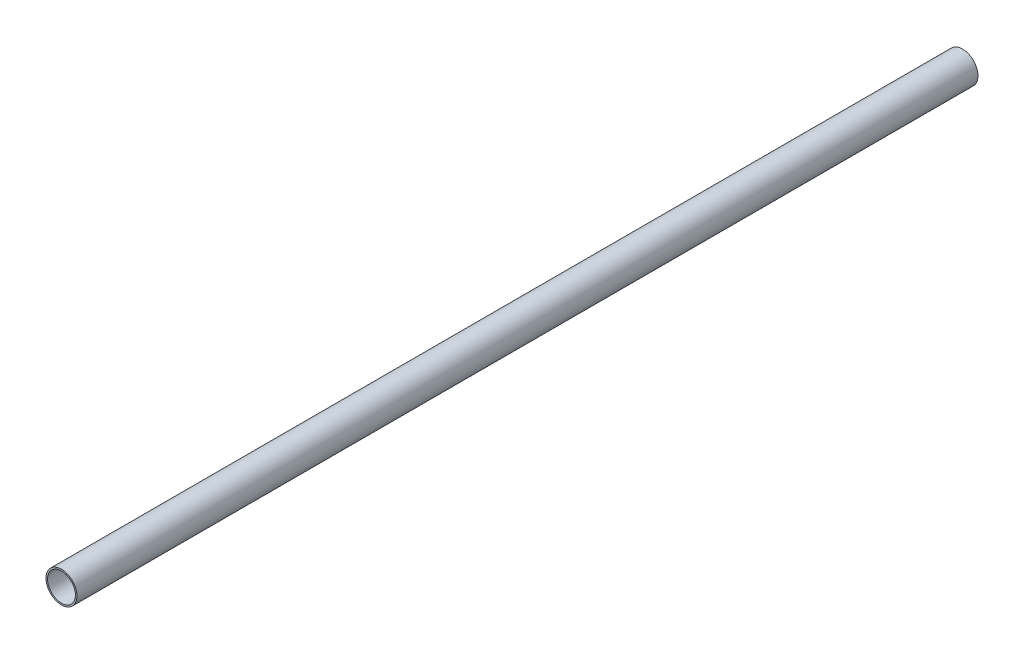
SolidWorks part; units mm, degrees
ref_plane "Front Plane" through (0, 0, 0) normal (0, 0, 1) x (1, 0, 0)
ref_plane "Top Plane" through (0, 0, 0) normal (0, 1, 0) x (1, 0, 0)
ref_plane "Right Plane" through (0, 0, 0) normal (1, 0, 0) x (0, 0, -1)
other "Configuration Table"
sketch "Sketch1" plane through (0, 0, 0) normal (0, 0, 1) x (1, 0, 0)
  circle A0 centre (0, 0) radius 13
  circle A1 centre (0, 0) radius 14.45
  dimension "D1" = 28.9
  dimension "D2" = 26
extrude "Boss-Extrude1" add sketch "Sketch1" along normal blind 840
